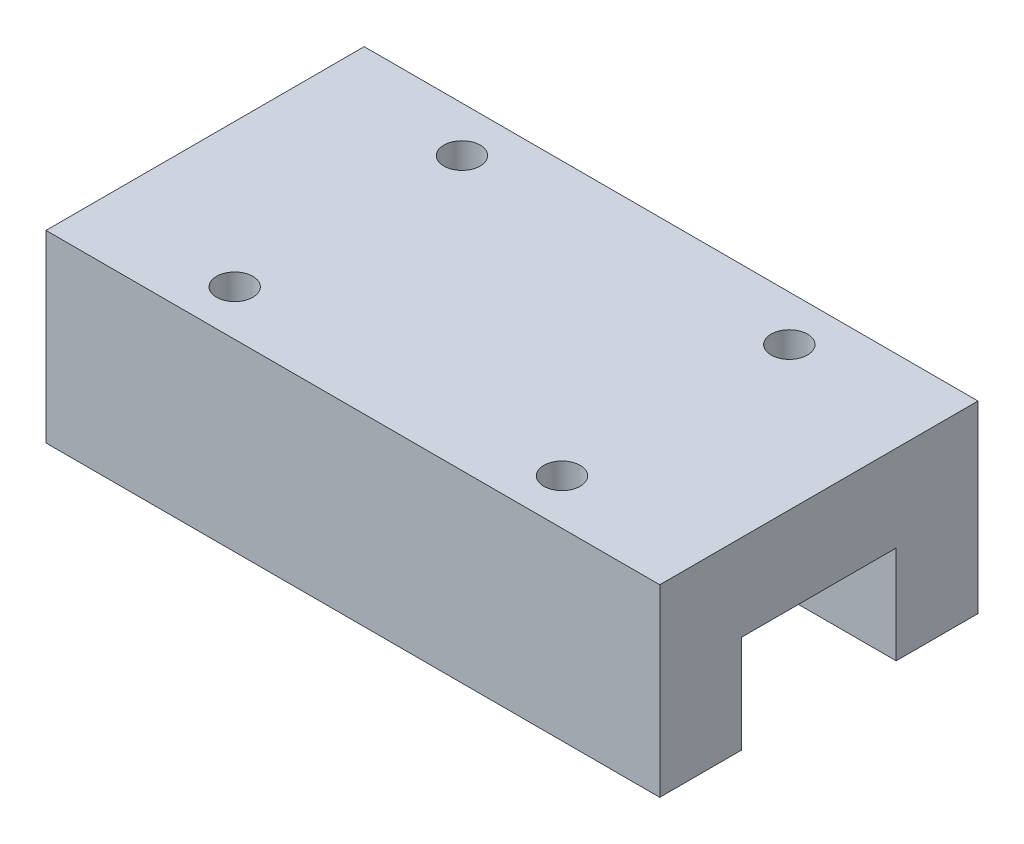
from build123d import *

# Parameters (mm, degrees)
SKETCH_1_W          = 135
SKETCH_1_H          = 70
EXTRUDE_1_DEPTH     = 40.5
SKETCH_2_W          = 135
SKETCH_2_H          = 34
CUT_EXTRUDE_1_DEPTH = 21.5
SKETCH_3_R          = 4
CUT_EXTRUDE_2_DEPTH = 16


with BuildPart() as part:
    # 草图1 → 拉伸1 (new body)
    with BuildSketch(Plane(origin=(0, 0, 0), x_dir=(1, 0, 0), z_dir=(0, 1, 0))):
        with Locations((67.5, 35)):
            Rectangle(SKETCH_1_W, SKETCH_1_H)
    extrude(amount=EXTRUDE_1_DEPTH)

    # 草图2 → 切除-拉伸1 (cut)
    with BuildSketch(Plane.XZ):
        with Locations((67.5, -35)):
            Rectangle(SKETCH_2_W, SKETCH_2_H)
    extrude(amount=-CUT_EXTRUDE_1_DEPTH, mode=Mode.SUBTRACT)

    # 草图3 → 切除-拉伸2 (cut)
    with BuildSketch(Plane(origin=(0, 40.5, 0), x_dir=(-1, 0, 0), z_dir=(0, 1, 0))):
        with Locations(Location((-103.5, -60, 0), (0, 0, 90))):
            Circle(SKETCH_3_R)
        with Locations(Location((-103.5, -10, 0), (0, 0, 90))):
            Circle(SKETCH_3_R)
        with Locations(Location((-31.5, -60, 0), (0, 0, 90))):
            Circle(SKETCH_3_R)
        with Locations(Location((-31.5, -10, 0), (0, 0, 90))):
            Circle(SKETCH_3_R)
    extrude(amount=-CUT_EXTRUDE_2_DEPTH, mode=Mode.SUBTRACT)


solid = part.part
